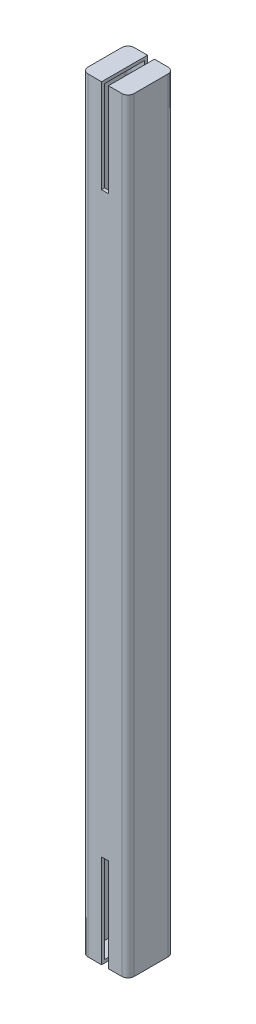
from build123d import *

# Parameters (mm, degrees)
BOSS_EXTRUDE1_DEPTH     = 998
CUT_EXTRUDE1_DEPTH      = 1001.251968256
CUT_EXTRUDE1_DEPTH_BACK = 1001.251968256
SKETCH2_W               = 9
SKETCH2_H               = 244
SKETCH3_W               = 21.5
SKETCH3_H               = 52
BOSS_EXTRUDE2_DEPTH     = 4
SKETCH4_W               = 21.5
SKETCH4_H               = 52
BOSS_EXTRUDE3_DEPTH     = 4


with BuildPart() as part:
    # Sketch1 → Boss-Extrude1 (new body)
    with BuildSketch(Plane(origin=(0, 0, 0), x_dir=(1, 0, 0), z_dir=(0, 1, 0))):
        with BuildLine():
            Line((-22, -30), (22, -30))
            ThreePointArc((22, -30), (27.656854249, -27.656854249), (30, -22))
            Line((30, -22), (30, 22))
            ThreePointArc((30, 22), (27.656854249, 27.656854249), (22, 30))
            Line((22, 30), (-22, 30))
            ThreePointArc((-22, 30), (-27.656854249, 27.656854249), (-30, 22))
            Line((-30, 22), (-30, -22))
            ThreePointArc((-30, -22), (-27.656854249, -27.656854249), (-22, -30))
        make_face()
        with BuildLine():
            Line((-22, 26), (22, 26))
            ThreePointArc((22, 26), (24.828427125, 24.828427125), (26, 22))
            Line((26, 22), (26, -22))
            ThreePointArc((26, -22), (24.828427125, -24.828427125), (22, -26))
            Line((22, -26), (-22, -26))
            ThreePointArc((-22, -26), (-24.828427125, -24.828427125), (-26, -22))
            Line((-26, -22), (-26, 22))
            ThreePointArc((-26, 22), (-24.828427125, 24.828427125), (-22, 26))
        make_face(mode=Mode.SUBTRACT)
    extrude(amount=BOSS_EXTRUDE1_DEPTH)

    # Sketch2 → Cut-Extrude1 (cut, two sides: drawn at the far end of the back side and taken through both)
    with BuildSketch(Plane.XY.offset(30).offset(-CUT_EXTRUDE1_DEPTH_BACK)):
        with Locations((0, 998)):
            Rectangle(SKETCH2_W, SKETCH2_H)
        Rectangle(SKETCH2_W, SKETCH2_H)
    extrude(amount=CUT_EXTRUDE1_DEPTH + CUT_EXTRUDE1_DEPTH_BACK, mode=Mode.SUBTRACT)

    # Sketch3 → Boss-Extrude2 (add)
    with BuildSketch(Plane(origin=(0, 998, 0), x_dir=(1, 0, 0), z_dir=(0, 1, 0))):
        with Locations((-15.25, 0)):
            Rectangle(SKETCH3_W, SKETCH3_H)
        with Locations((15.25, 0)):
            Rectangle(SKETCH3_W, SKETCH3_H)
    extrude(amount=-BOSS_EXTRUDE2_DEPTH)

    # Sketch4 → Boss-Extrude3 (add)
    with BuildSketch(Plane.XZ):
        with Locations((-15.25, 0)):
            Rectangle(SKETCH4_W, SKETCH4_H)
        with Locations((15.25, 0)):
            Rectangle(SKETCH4_W, SKETCH4_H)
    extrude(amount=-BOSS_EXTRUDE3_DEPTH)


solid = part.part
